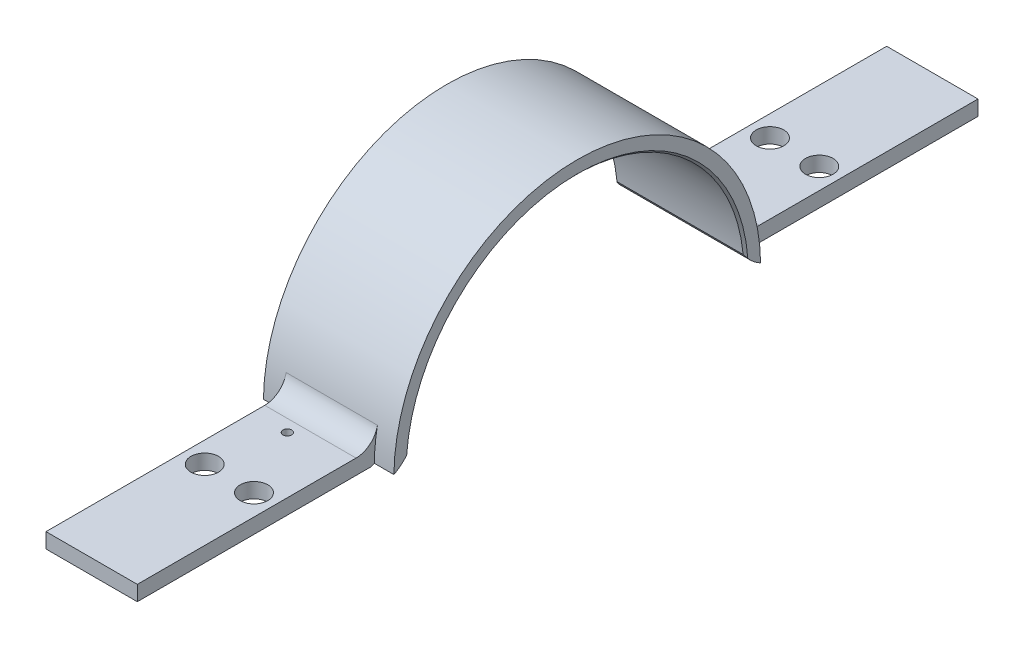
from build123d import *

# Parameters (mm, degrees)
BOSS_EXTRUDE1_DEPTH     = 90
FILLET1_R               = 30
FILLET2_R               = 55
CUT_EXTRUDE1_DEPTH      = 640.147087923
CUT_EXTRUDE1_DEPTH_BACK = 640.147087923
SKETCH2_R               = 233
CUT_EXTRUDE2_DEPTH      = 640.147087923
CUT_EXTRUDE2_DEPTH_BACK = 640.147087923
SKETCH3_W               = 1220
SKETCH3_H               = 21.2
CUT_EXTRUDE3_DEPTH      = 27
MIRROR2_COPY_1_DEPTH    = 27
CUT_EXTRUDE4_DEPTH      = 640.147087923
CUT_EXTRUDE4_DEPTH_BACK = 640.147087923
SKETCH5_R               = 19
SKETCH5_R_2             = 6
CHAMFER1_SIZE           = 3


with BuildPart() as part:
    # Sketch1 → Boss-Extrude1 (new, symmetric)
    with BuildSketch(Plane(origin=(0, 0, 0), x_dir=(0, 0, -1), z_dir=(1, 0, 0))):
        with BuildLine():
            Line((-580, 22), (-252.041663223, 22))
            ThreePointArc((-252.041663223, 22), (0, 253), (252.041663223, 22))
            Line((252.041663223, 22), (580, 22))
            Line((580, 22), (580, -3))
            Line((580, -3), (227.980262304, -3))
            ThreePointArc((227.980262304, -3), (0, 228), (-227.980262304, -3))
            Line((-227.980262304, -3), (-580, -3))
            Line((-580, -3), (-580, 22))
        make_face()
    extrude(amount=BOSS_EXTRUDE1_DEPTH, both=True)

    # Fillet1
    fillet1_edges = [part.edges().sort_by_distance(p)[0] for p in [
        (0, 22, 252.041663223),
        (0, 22, -252.041663223),
    ]]
    fillet(fillet1_edges, radius=FILLET1_R)

    # Fillet2
    fillet2_edges = [part.edges().sort_by_distance(p)[0] for p in [
        (0, -3, -227.980262304),
        (0, -3, 227.980262304),
    ]]
    fillet(fillet2_edges, radius=FILLET2_R)

    # Sketch2 → Cut-Extrude1 (cut, two sides: drawn at the far end of the back side and taken through both)
    with BuildSketch(Plane(origin=(0, 0, 0), x_dir=(0, 0, -1), z_dir=(1, 0, 0)).offset(-CUT_EXTRUDE1_DEPTH_BACK)):
        Circle(SKETCH2_R)
    extrude(amount=CUT_EXTRUDE1_DEPTH + CUT_EXTRUDE1_DEPTH_BACK, mode=Mode.SUBTRACT)

    # Sketch3 → Cut-Extrude2 (cut, two sides: drawn at the far end of the back side and taken through both)
    with BuildSketch(Plane(origin=(0, 0, 0), x_dir=(0, 0, -1), z_dir=(1, 0, 0)).offset(-CUT_EXTRUDE2_DEPTH_BACK)):
        with Locations((0, -9.4)):
            Rectangle(SKETCH3_W, SKETCH3_H)
    extrude(amount=CUT_EXTRUDE2_DEPTH + CUT_EXTRUDE2_DEPTH_BACK, mode=Mode.SUBTRACT)

    # Sketch4 → Cut-Extrude3 (cut)
    with BuildSketch(Plane(origin=(90, 0, 0), x_dir=(0, 0, -1), z_dir=(1, 0, 0))):
        with BuildLine():
            Line((-598.01008044, 50), (-248.01008044, 50))
            ThreePointArc((-248.01008044, 50), (-252.546221213, 15.14615962), (-252.208247288, -20))
            Line((-252.208247288, -20), (-598.01008044, -20))
            Line((-598.01008044, -20), (-598.01008044, 50))
        make_face()
    cut_extrude3 = extrude(amount=-CUT_EXTRUDE3_DEPTH, mode=Mode.SUBTRACT)

    # Mirror1: Cut-Extrude3 across plane
    add(cut_extrude3.mirror(Plane.XY), mode=Mode.SUBTRACT)

    # Mirror2: Cut-Extrude3 across plane
    add(cut_extrude3.mirror(Plane(origin=(0, 0, 0), x_dir=(0, 0, 1), z_dir=(1, 0, 0))), mode=Mode.SUBTRACT)

    # Mirror2 copy 1 sketch → Mirror2 copy 1 (cut)
    with BuildSketch(Plane.ZY.offset(90)):
        with BuildLine():
            Line((-598.01008044, 50), (-248.01008044, 50))
            ThreePointArc((-248.01008044, 50), (-252.546221213, 15.14615962), (-252.208247288, -20))
            Line((-252.208247288, -20), (-598.01008044, -20))
            Line((-598.01008044, -20), (-598.01008044, 50))
        make_face()
    extrude(amount=-MIRROR2_COPY_1_DEPTH, mode=Mode.SUBTRACT)

    # Sketch5 → Cut-Extrude4 (cut, two sides: drawn at the far end of the back side and taken through both)
    with BuildSketch(Plane(origin=(0, 0, 0), x_dir=(1, 0, 0), z_dir=(0, 1, 0)).offset(-CUT_EXTRUDE4_DEPTH_BACK)):
        with Locations(Location((34, -390, 0), (0, 0, 90))):
            Circle(SKETCH5_R)
        with Locations(Location((34, 390, 0), (0, 0, 90))):
            Circle(SKETCH5_R)
        with Locations(Location((-34, -390, 0), (0, 0, 90))):
            Circle(SKETCH5_R)
        with Locations(Location((-34, 390, 0), (0, 0, 90))):
            Circle(SKETCH5_R)
        with Locations(Location((-15, -295, 0), (0, 0, 90))):
            Circle(SKETCH5_R_2)
        with Locations(Location((15, 295, 0), (0, 0, 90))):
            Circle(SKETCH5_R_2)
    extrude(amount=CUT_EXTRUDE4_DEPTH + CUT_EXTRUDE4_DEPTH_BACK, mode=Mode.SUBTRACT)

    # Chamfer1
    chamfer1_edges = [part.edges().sort_by_distance(p)[0] for p in [
        (-90, 233, 0),
        (90, 233, 0),
    ]]
    chamfer(chamfer1_edges, length=CHAMFER1_SIZE)


solid = part.part
